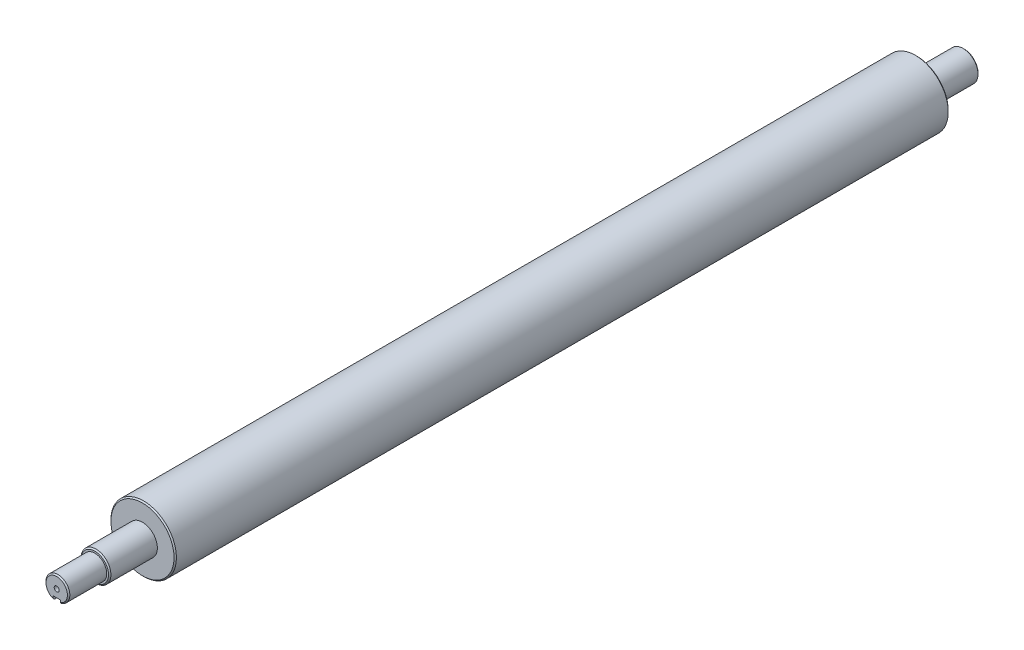
from build123d import *

# Parameters (mm, degrees)
SKETCH1_R             = 27.5
BOSS_EXTRUDE1_DEPTH   = 325
SKETCH2_R             = 12.5
BOSS_EXTRUDE2_DEPTH   = 40
CHAMFER1_SIZE         = 1
SKETCH3_R             = 10
BOSS_EXTRUDE3_DEPTH   = 32
CHAMFER2_SIZE         = 1
CUT_EXTRUDE1_START    = -6.5
CUT_EXTRUDE1_DEPTH    = 10
M5_TAPPED_HOLE1_D     = 4.2
M5_TAPPED_HOLE1_DEPTH = 12.4
M5_TAPPED_HOLE1_TIP   = 1.2618073


with BuildPart() as part:
    # Sketch1 → Boss-Extrude1 (new, symmetric)
    with BuildSketch(Plane.XY):
        Circle(SKETCH1_R)
    extrude(amount=BOSS_EXTRUDE1_DEPTH, both=True)

    # Sketch2 → Boss-Extrude2 (add)
    with BuildSketch(Plane.XY.offset(325)):
        Circle(SKETCH2_R)
    boss_extrude2 = extrude(amount=BOSS_EXTRUDE2_DEPTH)

    # Mirror1: Boss-Extrude2 across plane
    add(boss_extrude2.mirror(Plane.XY))

    # Chamfer1
    chamfer1_edges = [part.edges().sort_by_distance(p)[0] for p in [
        (-12.5, 0, -365),
        (-27.5, 0, -325),
        (-27.5, 0, 325),
        (-12.5, 0, 365),
    ]]
    chamfer(chamfer1_edges, length=CHAMFER1_SIZE)

    # Sketch3 → Boss-Extrude3 (add)
    with BuildSketch(Plane.XY.offset(365)):
        Circle(SKETCH3_R)
    extrude(amount=BOSS_EXTRUDE3_DEPTH)

    # Chamfer2
    chamfer2_edges = [part.edges().sort_by_distance(p)[0] for p in [
        (-10, 0, 397),
    ]]
    chamfer(chamfer2_edges, length=CHAMFER2_SIZE)

    # Sketch4 → Cut-Extrude1 (cut)
    with BuildSketch(Plane(origin=(0, 0, 0), x_dir=(1, 0, 0), z_dir=(0, 1, 0)).offset(CUT_EXTRUDE1_START)):
        with BuildLine():
            Line((-3, -424.5), (-3, -369.5))
            ThreePointArc((-3, -369.5), (0, -366.5), (3, -369.5))
            Line((3, -369.5), (3, -424.5))
            ThreePointArc((3, -424.5), (0, -427.5), (-3, -424.5))
        make_face()
    extrude(amount=-CUT_EXTRUDE1_DEPTH, mode=Mode.SUBTRACT)

    # M5 Tapped Hole1
    with Locations(Plane.XY.offset(397)):
        with Locations((0, 0)):
            Hole(M5_TAPPED_HOLE1_D / 2, depth=M5_TAPPED_HOLE1_DEPTH)
            with Locations((0, 0, -(M5_TAPPED_HOLE1_DEPTH + M5_TAPPED_HOLE1_TIP / 2))):  # 118° drill point
                Cone(0, M5_TAPPED_HOLE1_D / 2, M5_TAPPED_HOLE1_TIP, mode=Mode.SUBTRACT)


solid = part.part
